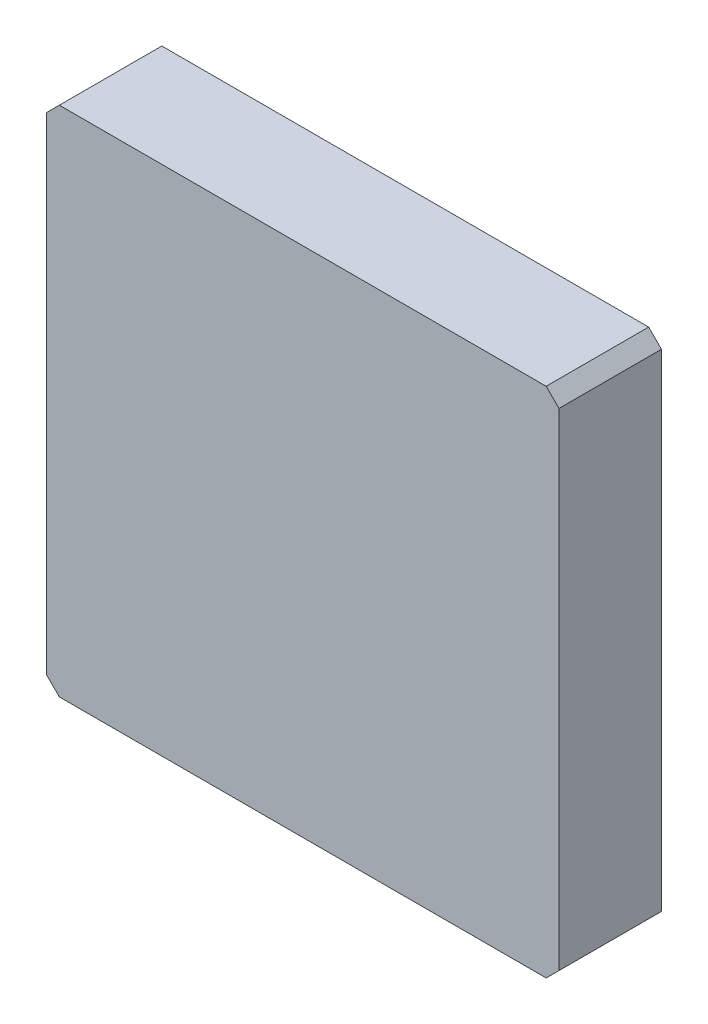
from build123d import *

# Parameters (mm, degrees)
SKETCH1_W           = 40
SKETCH1_H           = 40
BOSS_EXTRUDE1_DEPTH = 8
CHAMFER1_SIZE       = 1


with BuildPart() as part:
    # Sketch1 → Boss-Extrude1 (new body)
    with BuildSketch(Plane.XY):
        Rectangle(SKETCH1_W, SKETCH1_H)
    extrude(amount=BOSS_EXTRUDE1_DEPTH)

    # Chamfer1
    chamfer1_edges = [part.edges().sort_by_distance(p)[0] for p in [
        (20, -20, 4),
        (-20, -20, 4),
        (-20, 20, 4),
        (20, 20, 4),
    ]]
    chamfer(chamfer1_edges, length=CHAMFER1_SIZE)


solid = part.part
